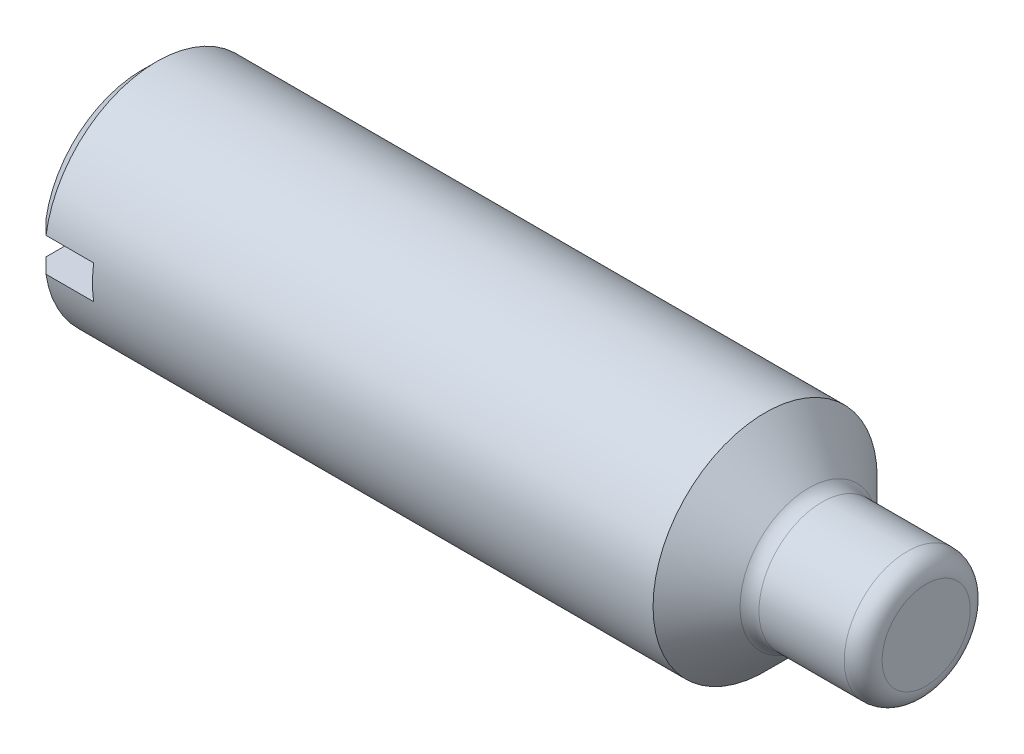
SolidWorks part; units mm, degrees
ref_plane "Front Plane" through (0, 0, 0) normal (0, 0, 1) x (1, 0, 0)
ref_plane "Top Plane" through (0, 0, 0) normal (0, 1, 0) x (1, 0, 0)
ref_plane "Right Plane" through (0, 0, 0) normal (1, 0, 0) x (0, 0, -1)
sketch "Dimensioned Sketch" plane through (0, 0, 0) normal (0, 0, 1) x (1, 0, 0)
  line L0 (0, 0) -> (14, 0) construction
  line L1 (14, 0) -> (14, 2.25) construction
  line L2 (0, 0) -> (0, 3.464) construction
  point P5 (0.6, 0)
  point P6 (12, 0)
  point P7 (1.12, 0)
  point P8 (13.3, 0)
  point P9 (4, 0)
  dimension "l" = 14
  dimension "dp" = 2.25
  dimension "df" = 3.464
  dimension "t" = 1.12
  dimension "n" = 0.6
  dimension "z" = 2
  dimension "P" = 0.7
  dimension "d" = 4
sketch "Sketch3" plane through (0, 0, 0) normal (0, 0, 1) x (1, 0, 0)
  line L0 (0, 0) -> (0, 1.732)
  line L1 (0, 1.732) -> (0.268, 2)
  line L2 (0.268, 2) -> (11.125, 2)
  line L3 (11.125, 2) -> (12, 1.125)
  line L4 (12, 1.125) -> (14, 1.125)
  line L5 (14, 1.125) -> (14, 0)
  line L6 (0, 0) -> (14, 0) construction
  line L7 (14, 0) -> (0, 0)
  line L8 (-1.4251, 0) -> (7.1744, 0) construction
  dimension "D1" = 45
  dimension "df" = 3.464
  dimension "D2" = 45
  dimension "d" = 4
  dimension "dp" = 2.25
  dimension "z" = 2
  dimension "l" = 14
revolve "Base-Revolve" add sketch "Sketch3"
cosmetic thread "Cosmetic Thread1"
extrude "Cut-Extrude1" cut sketch "Sketch4" against normal mid plane 100
sketch "Sketch4" plane through (0, 0, 0) normal (0, 0, 1) x (1, 0, 0)
  line L1 (0, 0.3) -> (1.12, 0.3)
  line L2 (0, 0.3) -> (0, -0.3)
  line L3 (0, -0.3) -> (1.12, -0.3)
  line L4 (1.12, 0.3) -> (1.12, -0.3)
  dimension "n" = 0.6
  dimension "t" = 1.12
fillet "Fillet1" radius 0.3375 2 edges at (12, 0, 1.125) (14, 0, 1.125)
